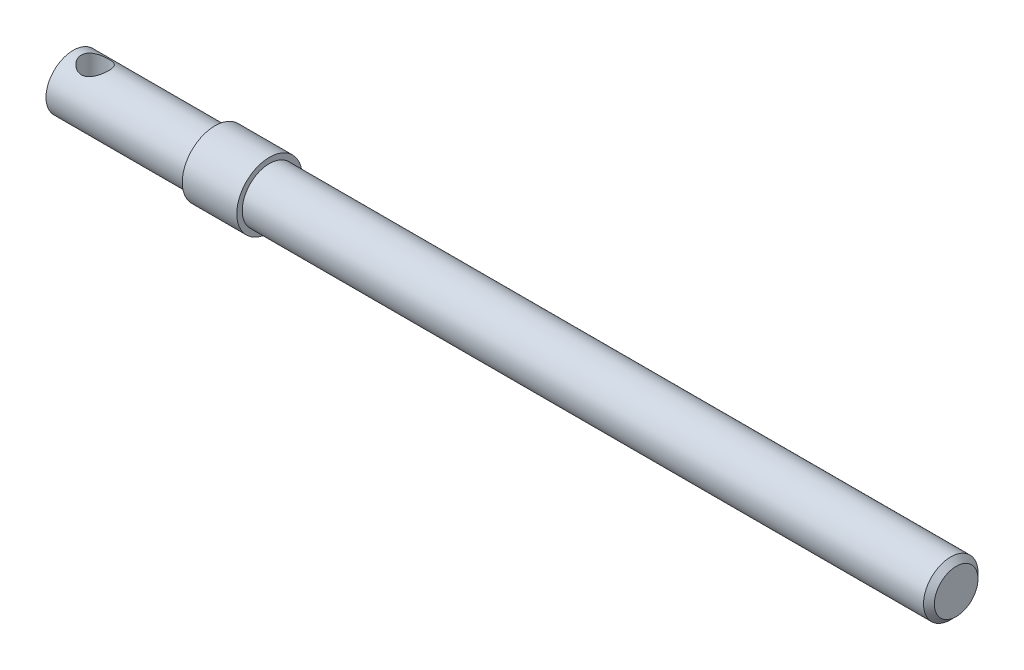
from build123d import *

# Parameters (mm, degrees)
SKETCH1_W                      = 5
SKETCH1_H                      = 3
SKETCH2_R                      = 2.5
BOSS_EXTRUDE1_DEPTH            = 13
BOSS_EXTRUDE2_START            = 63
SKETCH3_R                      = 2.5
BOSS_EXTRUDE2_DEPTH            = 63
F_2_5_2_5_DIAMETER_HOLE1_D     = 2.5
F_2_5_2_5_DIAMETER_HOLE1_DEPTH = 5.5
CHAMFER1_SIZE                  = 0.5


with BuildPart() as part:
    # Sketch1 → Revolve1 (revolve)
    with BuildSketch(Plane(origin=(0, 0, 0), x_dir=(-1, 0, 0), z_dir=(0, 0, -1)), mode=Mode.PRIVATE) as revolve1_sk:
        with Locations((-15.5, 1.5)):
            Rectangle(SKETCH1_W, SKETCH1_H)
    revolve(revolve1_sk.sketch.rotate(Axis((18, 0, 0), (-1, 0, 0)), 270), axis=Axis((18, 0, 0), (-1, 0, 0)))

    # Sketch2 → Boss-Extrude1 (add)
    with BuildSketch(Plane.ZY.offset(-13)):
        with Locations(Location((0, 0, 0), (0, 0, 180))):
            Circle(SKETCH2_R)
    extrude(amount=BOSS_EXTRUDE1_DEPTH)

    # Sketch3 → Boss-Extrude2 (add)
    with BuildSketch(Plane(origin=(18, 0, 0), x_dir=(0, 0, -1), z_dir=(1, 0, 0)).offset(BOSS_EXTRUDE2_START)):
        Circle(SKETCH3_R)
    extrude(amount=-BOSS_EXTRUDE2_DEPTH)

    # Ø2.5 (2.5) Diameter Hole1
    with Locations(Plane(origin=(2, -2.5, 0), x_dir=(-1, 0, 0), z_dir=(0, -1, 0))):
        with Locations((0, 0)):
            Hole(F_2_5_2_5_DIAMETER_HOLE1_D / 2, depth=F_2_5_2_5_DIAMETER_HOLE1_DEPTH)

    # Chamfer1
    chamfer1_edges = [part.edges().sort_by_distance(p)[0] for p in [
        (81, 0, 2.5),
    ]]
    chamfer(chamfer1_edges, length=CHAMFER1_SIZE)


solid = part.part
